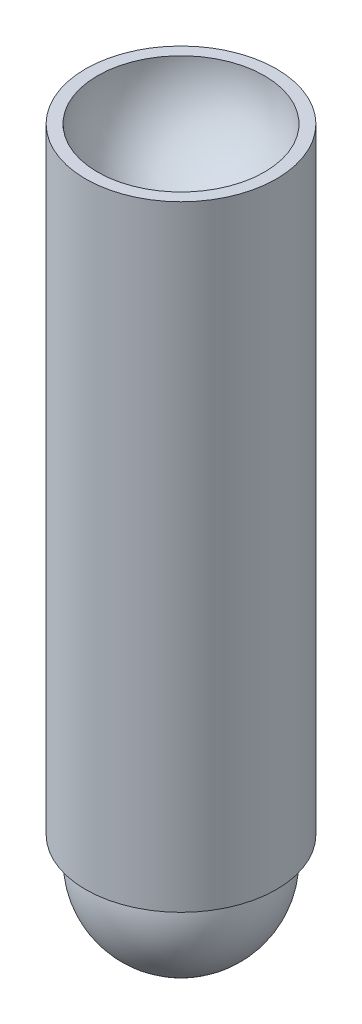
SolidWorks part; units mm, degrees
ref_plane "Front Plane" through (0, 0, 0) normal (0, 0, 1) x (1, 0, 0)
ref_plane "Top Plane" through (0, 0, 0) normal (0, 1, 0) x (1, 0, 0)
ref_plane "Right Plane" through (0, 0, 0) normal (1, 0, 0) x (0, 0, -1)
other "Configuration Table"
sketch "Sketch1" plane through (0, 0, 0) normal (0, 0, 1) x (1, 0, 0)
  line L0 (0, 0) -> (0, 60) construction
  line L1 (-2, 0) -> (-2, 53.2918)
  line L2 (-7, 60) -> (-8, 60)
  line L3 (-8, 60) -> (-8, 8.3924)
  line L5 (-2, 0) -> (-2.5, 0)
  line L6 (-8, 8.3924) -> (-6.75, 8.3924)
  arc A0 (-2, 53.2918) -> (-7, 60) centre (0, 60) cw
  arc A2 (-6.75, 8.3924) -> (-2.5, 0) centre (0, 6.5383) ccw
  dimension "D6" = 7
  dimension "D7" = 14
  dimension "D1" = 8
  dimension "D2" = 2
  dimension "D3" = 1
  dimension "D4" = 60
  dimension "D5" = 0.5
  dimension "D8" = 1.25
revolve "Revolve2" add sketch "Sketch1" angle 360 about L0
